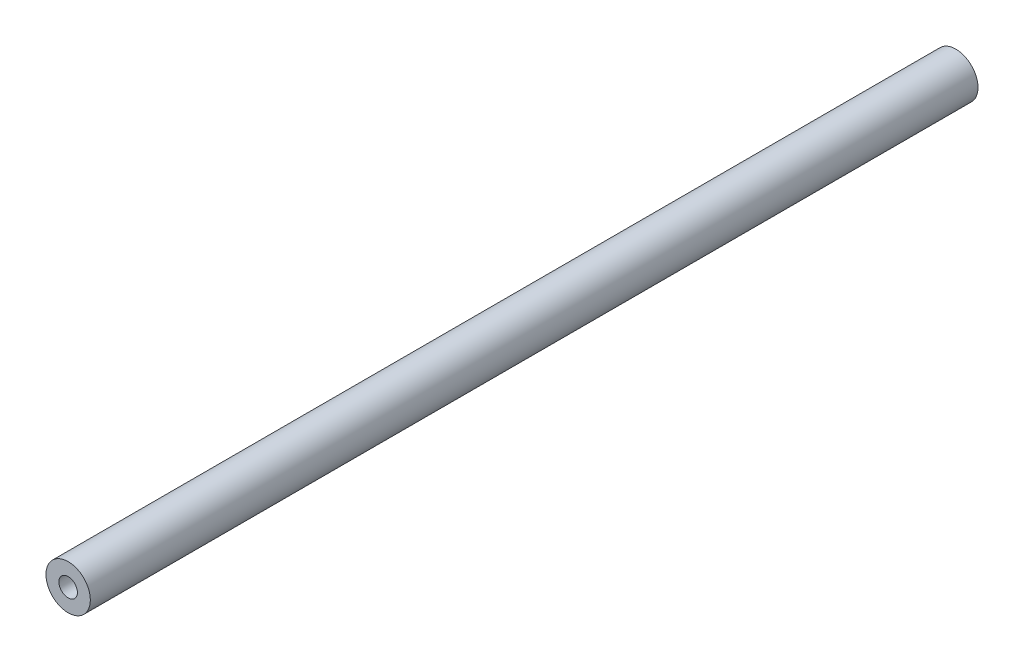
SolidWorks part; units mm, degrees
ref_plane "Front Plane" through (0, 0, 0) normal (0, 0, 1) x (1, 0, 0)
ref_plane "Top Plane" through (0, 0, 0) normal (0, 1, 0) x (1, 0, 0)
ref_plane "Right Plane" through (0, 0, 0) normal (1, 0, 0) x (0, 0, -1)
sketch "Sketch1" plane through (0, 0, 0) normal (0, 0, 1) x (1, 0, 0)
  circle A0 centre (0, 0) radius 3
  dimension "D1" = 6
extrude "Boss-Extrude1" add sketch "Sketch1" along normal blind 120
sketch "Sketch2" plane through (0, 0, 120) normal (0, 0, 1) x (1, 0, 0)
  circle A0 centre (0, 0) radius 6
  dimension "D1" = 12
hole_wizard "M3 Tapped Hole1" positions "Sketch3" profile "Sketch4" tap size "M3" standard "GB"
sketch "Sketch3" plane through (0, 0, 120) normal (0, 0, 1) x (1, 0, 0)
  point P0 (0, 0)
sketch "Sketch4" plane through (0, 0, 120) normal (1, 0, 0) x (0, -1, 0)
  line L0 (0, 0) -> (0, 9.2511)
  line L1 (0, 9.2511) -> (1.25, 8.5)
  line L2 (1.25, 8.5) -> (1.25, 0)
  line L5 (1.25, 0) -> (0, 0)
  line L10 (0, 9.2511) -> (-1.25, 8.5) construction
  line L11 (0, -6.35) -> (0, 107.95) construction
  dimension "螺纹孔钻头直径" = 2.5
  dimension "螺纹孔钻头深度" = 8.5
  dimension "导头角度" = 118
cosmetic thread "Cosmetic thread 1" parameters "D1"=6, "D2"=3
hole_wizard "M3 Tapped Hole2" positions "Sketch5" profile "Sketch6" tap size "M3" standard "GB"
sketch "Sketch5" plane through (0, 0, 0) normal (0, 0, -1) x (-1, 0, 0)
  point P0 (0, 0)
sketch "Sketch6" plane through (0, 0, 0) normal (1, 0, 0) x (0, 1, 0)
  line L0 (0, 0) -> (0, 9.2511)
  line L1 (0, 9.2511) -> (1.25, 8.5)
  line L2 (1.25, 8.5) -> (1.25, 0)
  line L5 (1.25, 0) -> (0, 0)
  line L10 (0, 9.2511) -> (-1.25, 8.5) construction
  line L11 (0, -6.35) -> (0, 107.95) construction
  dimension "螺纹孔钻头直径" = 2.5
  dimension "螺纹孔钻头深度" = 8.5
  dimension "导头角度" = 118
cosmetic thread "Cosmetic thread 2" parameters "D1"=6, "D2"=3
